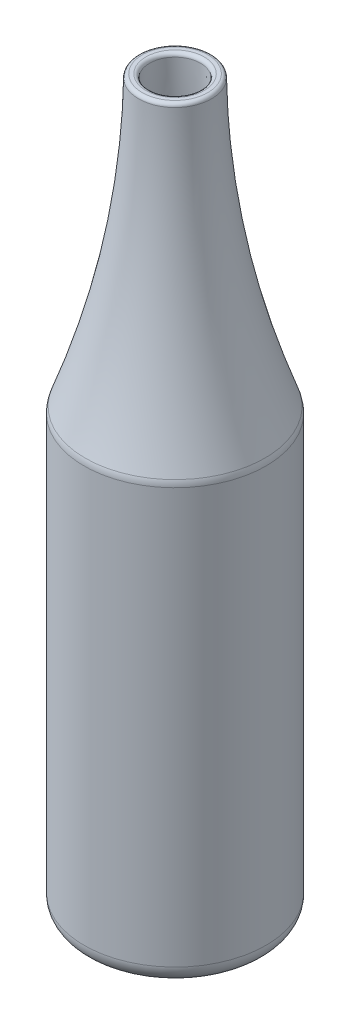
from build123d import *

# Parameters (mm, degrees)
SHELL1_T  = -3
FILLET1_R = 5
FILLET2_R = 1


with BuildPart() as part:
    # Sketch1 → Revolve1 (revolve)
    with BuildSketch(Plane.XY, mode=Mode.PRIVATE) as revolve1_sk:
        with BuildLine():
            Line((-93.039279644, 135.747175363), (-93.039279644, -64.252824637))
            Line((-93.039279644, -64.252824637), (-118.039279644, -64.252824637))
            Line((-118.039279644, -64.252824637), (-118.039279644, 55.747175363))
            add(Edge.make_bspline(
                [(-118.039279644, 55.747175363), (-103.478005536, 95.090899145), (-103.039279644, 135.747175363)],
                knots=[0, 0, 0, 0.941503214, 0.941503214, 0.941503214], degree=2))
            Line((-103.039279644, 135.747175363), (-93.039279644, 135.747175363))
        make_face()
    revolve(revolve1_sk.sketch.rotate(Axis((-93.039279644, 135.747175363, 0), (0, -1, 0)), 270), axis=Axis((-93.039279644, 135.747175363, 0), (0, -1, 0)))

    # Shell1
    shell1_openings = [part.faces().sort_by_distance(p)[0] for p in [
        (-93.039279644, 135.747175363, 0),
    ]]
    offset(amount=SHELL1_T, openings=shell1_openings, kind=Kind.INTERSECTION)

    # Fillet1
    fillet1_edges = [part.edges().sort_by_distance(p)[0] for p in [
        (-93.039279644, 55.747175363, -25),
        (-93.039279644, -64.252824637, -25),
    ]]
    fillet(fillet1_edges, radius=FILLET1_R)

    # Fillet2
    fillet2_edges = [part.edges().sort_by_distance(p)[0] for p in [
        (-93.039279644, 135.747175363, -6.999825357),
        (-93.039279644, 135.747175363, -10),
    ]]
    fillet(fillet2_edges, radius=FILLET2_R)


solid = part.part
